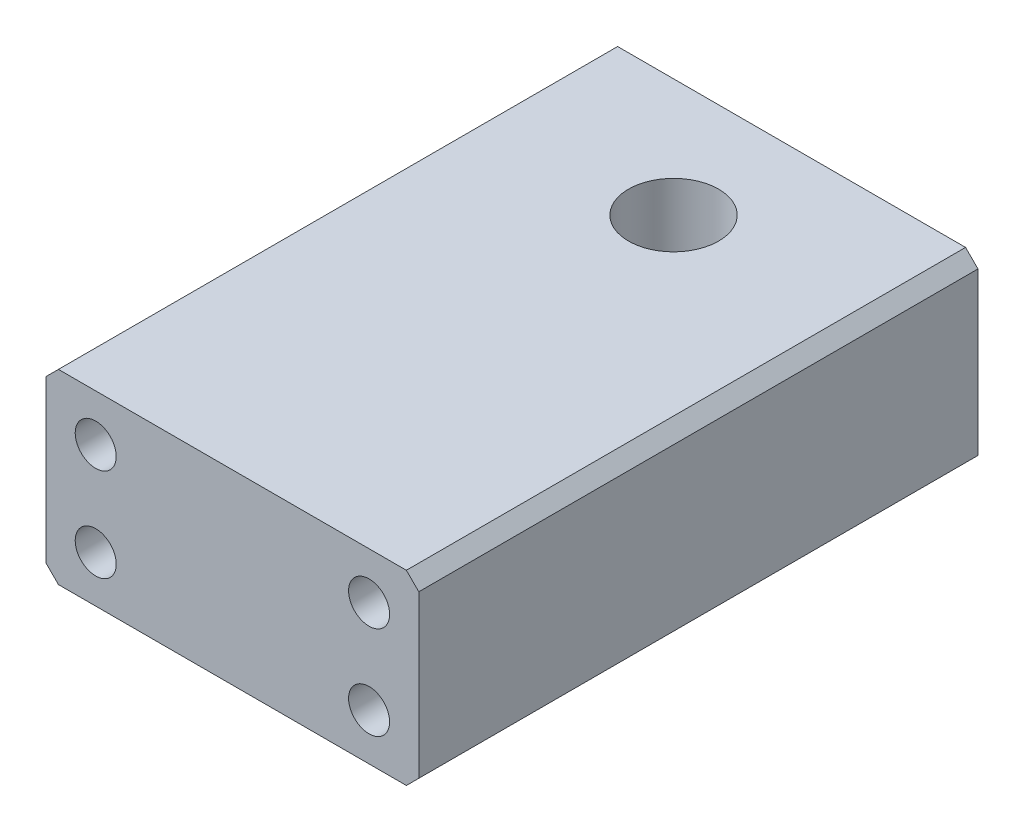
from build123d import *

# Parameters (mm, degrees)
SKETCH_1_W                   = 60
SKETCH_1_H                   = 30
EXTRUDE_1_DEPTH              = 90
M16X1_5_1_D                  = 14.5
HOLE_WIZARD_M6_1_D           = 6.6
HOLE_WIZARD_M6_1_CBORE_D     = 11
HOLE_WIZARD_M6_1_CBORE_DEPTH = 30
CHAMFER_1_SIZE               = 2


with BuildPart() as part:
    # 草图1 → 凸台-拉伸1 (new body)
    with BuildSketch(Plane.XY):
        Rectangle(SKETCH_1_W, SKETCH_1_H)
    extrude(amount=EXTRUDE_1_DEPTH)

    # M16x1.5 螺纹孔1 (through all)
    with Locations(Plane(origin=(0, -15, 0), x_dir=(-1, 0, 0), z_dir=(0, -1, 0))):
        with Locations((0, -19)):
            Hole(M16X1_5_1_D / 2)

    # M6 六角凹头螺钉的柱形沉头孔1 (through all)
    with Locations(Plane(origin=(0, 0, 0), x_dir=(-1, 0, 0), z_dir=(0, 0, -1))):
        with Locations((22, -7.5), (22, 7.5), (-22, 7.5), (-22, -7.5)):
            CounterBoreHole(HOLE_WIZARD_M6_1_D / 2, HOLE_WIZARD_M6_1_CBORE_D / 2, HOLE_WIZARD_M6_1_CBORE_DEPTH)

    # 倒角1
    chamfer_1_edges = [part.edges().sort_by_distance(p)[0] for p in [
        (30, -15, 45),
        (-30, -15, 45),
        (-30, 15, 45),
        (30, 15, 45),
    ]]
    chamfer(chamfer_1_edges, length=CHAMFER_1_SIZE)


solid = part.part
